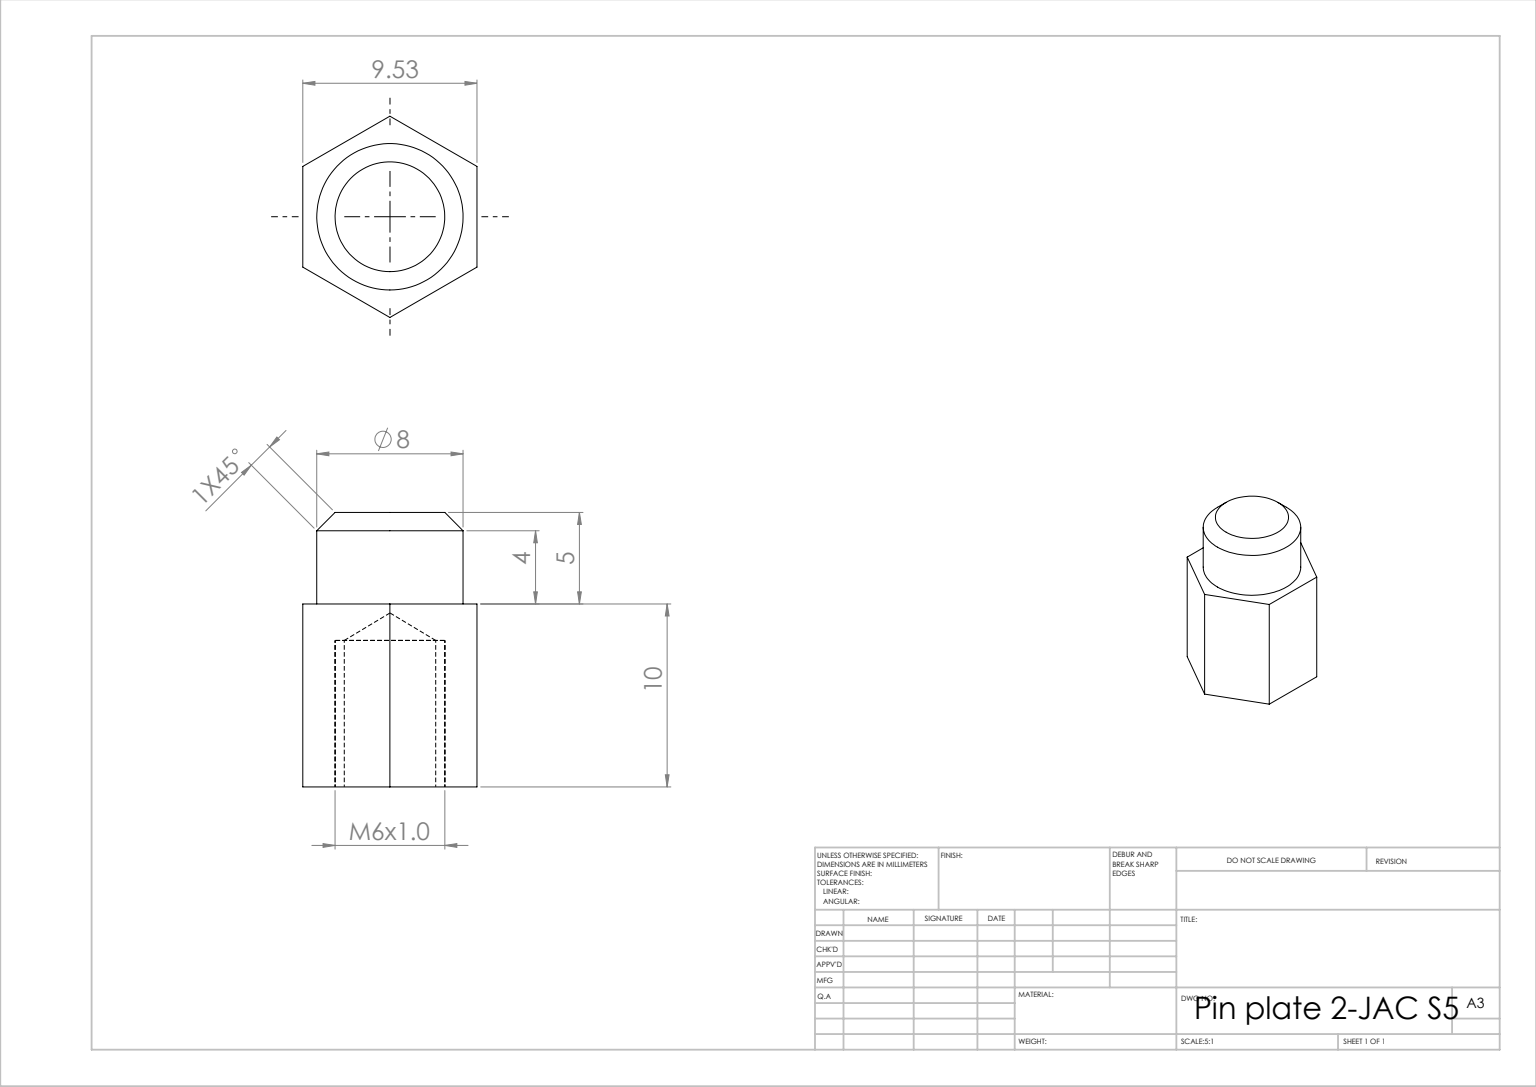
SolidWorks part; units mm, degrees
ref_plane "Front Plane" through (0, 0, 0) normal (0, 0, 1) x (1, 0, 0)
ref_plane "Top Plane" through (0, 0, 0) normal (0, 1, 0) x (1, 0, 0)
ref_plane "Right Plane" through (0, 0, 0) normal (1, 0, 0) x (0, 0, -1)
sketch "Sketch1" plane through (0, 0, 0) normal (0, 1, 0) x (1, 0, 0)
  line L1 (0, 5.5) -> (-4.7631, 2.75)
  line L2 (-4.7631, 2.75) -> (-4.7631, -2.75)
  line L3 (-4.7631, -2.75) -> (0, -5.5)
  line L4 (0, -5.5) -> (4.7631, -2.75)
  line L5 (4.7631, -2.75) -> (4.7631, 2.75)
  line L6 (4.7631, 2.75) -> (0, 5.5)
  circle A0 centre (0, 0) radius 4.7631 construction
  dimension "D1" = 11
extrude "Boss-Extrude1" add sketch "Sketch1" along normal mid plane 10
sketch "Sketch3" plane through (0, 5, 0) normal (0, 1, 0) x (1, 0, 0)
  circle A0 centre (0, 0) radius 4
  dimension "D1" = 8
extrude "Boss-Extrude2" add sketch "Sketch3" along normal blind 5
chamfer "Chamfer1" distance 1 angle 45 1 edges at (0, 10, 4)
hole_wizard "M6x1.0 Tapped Hole2" positions "3DSketch14" profile "Sketch19" tap size "M6x1.0" standard "ANSI Metric"
sketch3d "3DSketch14"
  point P0 (0, 0, 0)
  point P3 (0, 0, 0)
  point P5 (0, -5, 0.0001)
sketch "Sketch19" plane through (0, -5, 0.0001) normal (1, 0, 0) x (0, 0, -1)
  line L0 (0, 0) -> (0, 9.5022)
  line L1 (0, 9.5022) -> (2.5, 8)
  line L2 (2.5, 8) -> (2.5, 0)
  line L5 (2.5, 0) -> (0, 0)
  line L10 (0, 9.5022) -> (-2.5, 8) construction
  line L11 (0, -6.35) -> (0, 107.95) construction
  dimension "Tap Drill Dia." = 5
  dimension "Tap Drill Depth" = 8
  dimension "Drill Angle" = 118
cosmetic thread "Hole Thread5" parameters "D1"=8, "D2"=6
cosmetic thread "Hole Thread6" parameters "D1"=8, "D2"=6
cosmetic thread "Hole Thread7" parameters "D1"=8, "D2"=6
